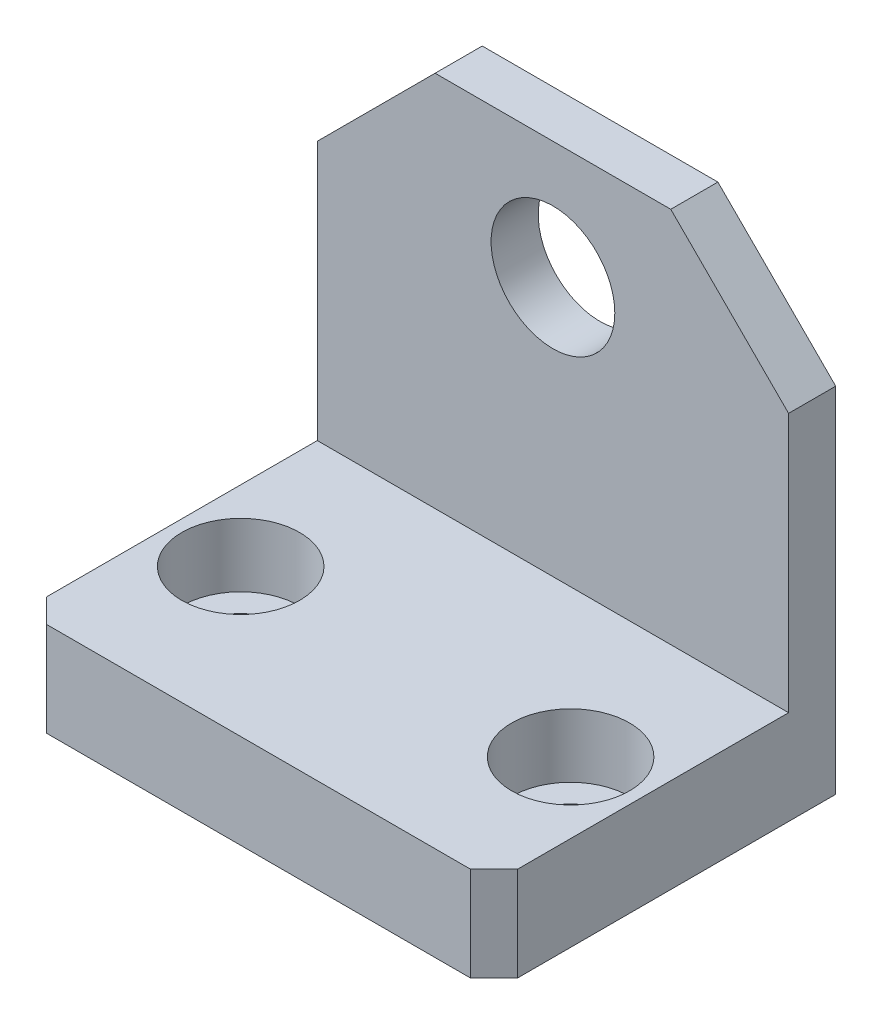
from build123d import *

# Parameters (mm, degrees)
SKETCH2_W                                           = 40
SKETCH2_H                                           = 40
BOSS_EXTRUDE1_DEPTH                                 = 4
SKETCH3_W                                           = 40
SKETCH3_H                                           = 8
BOSS_EXTRUDE2_DEPTH                                 = 25
SKETCH4_R                                           = 5.25
CUT_EXTRUDE1_DEPTH                                  = 25
CHAMFER1_SIZE                                       = 10
CBORE_FOR_M5_HEX_SOCKET_HEAD_CAP_SCREW1_D           = 5.5
CBORE_FOR_M5_HEX_SOCKET_HEAD_CAP_SCREW1_CBORE_D     = 10
CBORE_FOR_M5_HEX_SOCKET_HEAD_CAP_SCREW1_CBORE_DEPTH = 5.4
CHAMFER2_SIZE                                       = 2


with BuildPart() as part:
    # Sketch2 → Boss-Extrude1 (new body)
    with BuildSketch(Plane.XY):
        Rectangle(SKETCH2_W, SKETCH2_H)
    extrude(amount=BOSS_EXTRUDE1_DEPTH)

    # Sketch3 → Boss-Extrude2 (add)
    with BuildSketch(Plane.XY.offset(4)):
        with Locations((0, -16)):
            Rectangle(SKETCH3_W, SKETCH3_H)
    extrude(amount=BOSS_EXTRUDE2_DEPTH)

    # Sketch4 → Cut-Extrude1 (cut)
    with BuildSketch(Plane.XY.offset(4)):
        with Locations((0, 10)):
            Circle(SKETCH4_R)
    extrude(amount=-CUT_EXTRUDE1_DEPTH, mode=Mode.SUBTRACT)

    # Chamfer1
    chamfer1_edges = [part.edges().sort_by_distance(p)[0] for p in [
        (20, 20, 2),
        (-20, 20, 2),
    ]]
    chamfer(chamfer1_edges, length=CHAMFER1_SIZE)

    # CBORE for M5 Hex Socket Head Cap Screw1 (through all)
    with Locations(Plane(origin=(0, -12, 0), x_dir=(1, 0, 0), z_dir=(0, 1, 0))):
        with Locations((-14, -16.5), (14, -16.5)):
            CounterBoreHole(CBORE_FOR_M5_HEX_SOCKET_HEAD_CAP_SCREW1_D / 2, CBORE_FOR_M5_HEX_SOCKET_HEAD_CAP_SCREW1_CBORE_D / 2, CBORE_FOR_M5_HEX_SOCKET_HEAD_CAP_SCREW1_CBORE_DEPTH)

    # Chamfer2
    chamfer2_edges = [part.edges().sort_by_distance(p)[0] for p in [
        (20, -16, 29),
        (-20, -16, 29),
    ]]
    chamfer(chamfer2_edges, length=CHAMFER2_SIZE)


solid = part.part
